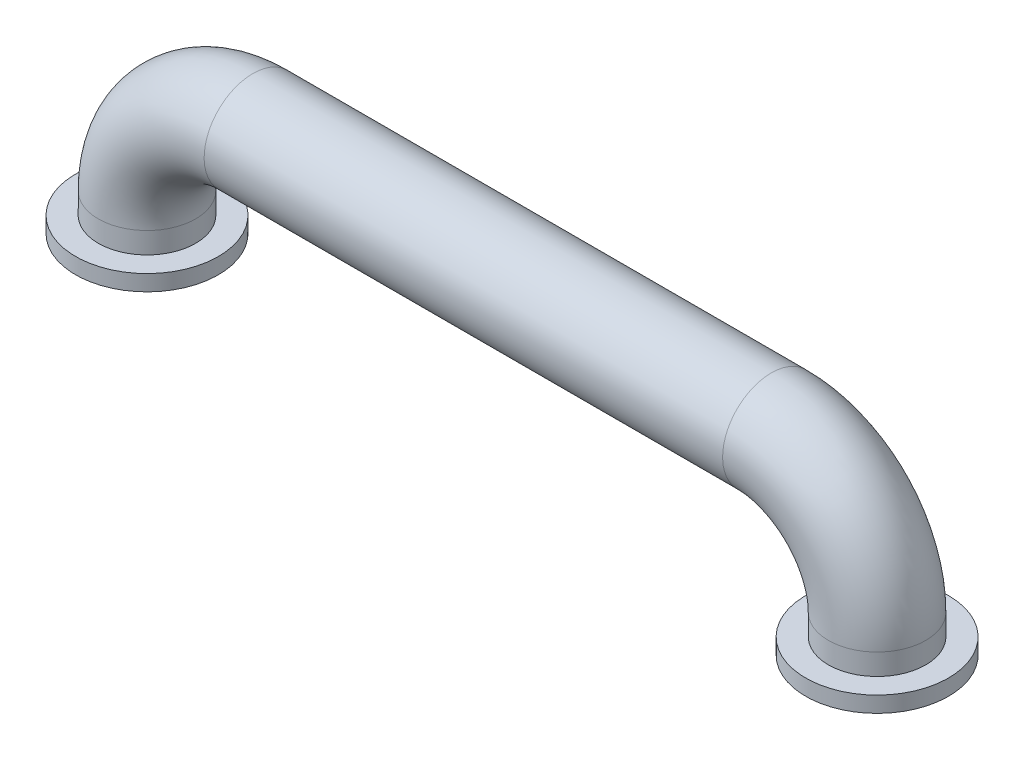
SolidWorks part; units mm, degrees
material "普通碳钢"
ref_plane "Front Plane" through (0, 0, 0) normal (0, 0, 1) x (1, 0, 0)
ref_plane "Top Plane" through (0, 0, 0) normal (0, 1, 0) x (1, 0, 0)
ref_plane "Right Plane" through (0, 0, 0) normal (1, 0, 0) x (0, 0, -1)
sketch "Sketch2" plane through (0, 0, 0) normal (0, 1, 0) x (1, 0, 0)
  circle A0 centre (0, 0) radius 46
  circle A1 centre (0, 0) radius 40
  dimension "D1" = 80
  dimension "D2" = 92
sketch "Sketch3" plane through (0, 0, 0) normal (0, 0, 1) x (1, 0, 0)
  line L0 (0, 0) -> (0, 20)
  line L1 (100, 120) -> (590, 120)
  line L2 (690, 20) -> (690, 0)
  arc A0 (590, 120) -> (690, 20) centre (590, 20) cw
  arc A1 (0, 20) -> (100, 120) centre (100, 20) cw
  point P7 (690, 120)
  point P10 (0, 120)
  dimension "D4" = 100
  dimension "D1" = 120
  dimension "D2" = 690
  dimension "D3" = 120
sweep "Sweep1" add profiles "Sketch2" path "Sketch3"
sketch "Sketch4" plane through (0, 0, 0) normal (0, -1, 0) x (-1, 0, 0)
  circle A0 centre (0, 0) radius 67.5
  circle A1 centre (0, 0) radius 40
  circle A2 centre (-690, 0) radius 40
  circle A3 centre (-690, 0) radius 67.5
  dimension "D1" = 135
  dimension "D2" = 135
extrude "Boss-Extrude1" add sketch "Sketch4" along normal blind 15
sketch "Sketch5" plane through (0, -15, 0) normal (0, -1, 0) x (-1, 0, 0)
  line L0 (0, 0) -> (0, -67.5) construction
  circle A0 centre (0, 0) radius 67.5 construction
